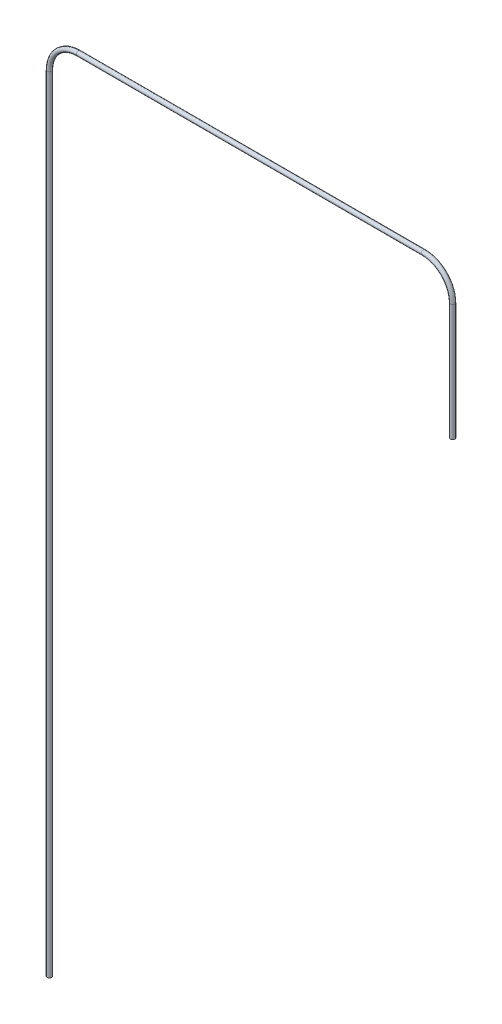
from build123d import *

# Parameters (mm, degrees)
SKETCH2_R = 3.25


with BuildPart() as part:
    # Sweep1: sweep along a path in Sketch1
    with BuildLine(Plane.XY) as sweep1_path:
        Line((0, 0), (0, 1133))
        ThreePointArc((0, 1133), (12.30151519, 1162.69848481), (42, 1175))
        Line((42, 1175), (540, 1175))
        ThreePointArc((540, 1175), (569.69848481, 1162.69848481), (582, 1133))
        Line((582, 1133), (582, 964.056768559))
    # Sketch2 → Sweep1 (sweep)
    with BuildSketch(Plane(origin=(0, 0, 0), x_dir=(1, 0, 0), z_dir=(0, 1, 0))):
        Circle(SKETCH2_R)
    sweep(path=sweep1_path.line)


solid = part.part
